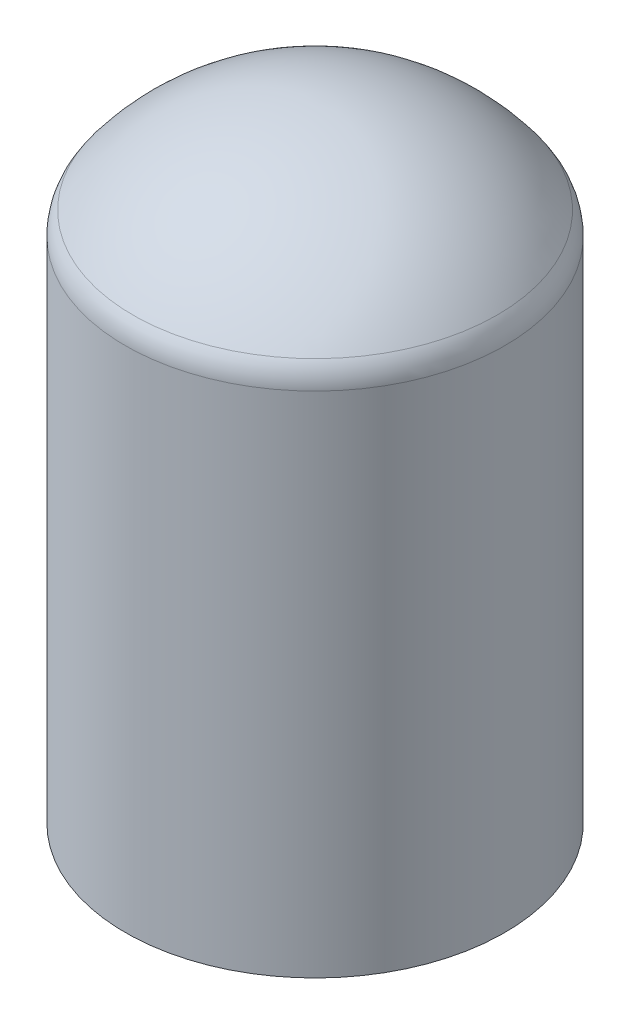
SolidWorks part; units mm, degrees
ref_plane "Front Plane" through (0, 0, 0) normal (0, 0, 1) x (1, 0, 0)
ref_plane "Top Plane" through (0, 0, 0) normal (0, 1, 0) x (1, 0, 0)
ref_plane "Right Plane" through (0, 0, 0) normal (1, 0, 0) x (0, 0, -1)
sketch "Sketch1" plane through (0, 0, 0) normal (0, 0, 1) x (1, 0, 0)
  line L0 (0, 0) -> (0, 700)
  line L2 (250, 685.8312) -> (250, 0)
  line L3 (250, 0) -> (0, 0)
  line L4 (0, 700) -> (0, 820)
  arc A1 (250, 685.8312) -> (0, 820) centre (0, 520) ccw
  dimension "D3" = 120
  dimension "D4" = 300
  dimension "D1" = 250
  dimension "D2" = 700
revolve "Revolve1" add sketch "Sketch1" angle 360 about L0
fillet "Fillet1" radius 50 1 edges at (0, 685.8312, -250)
shell "Shell1" thickness 70
